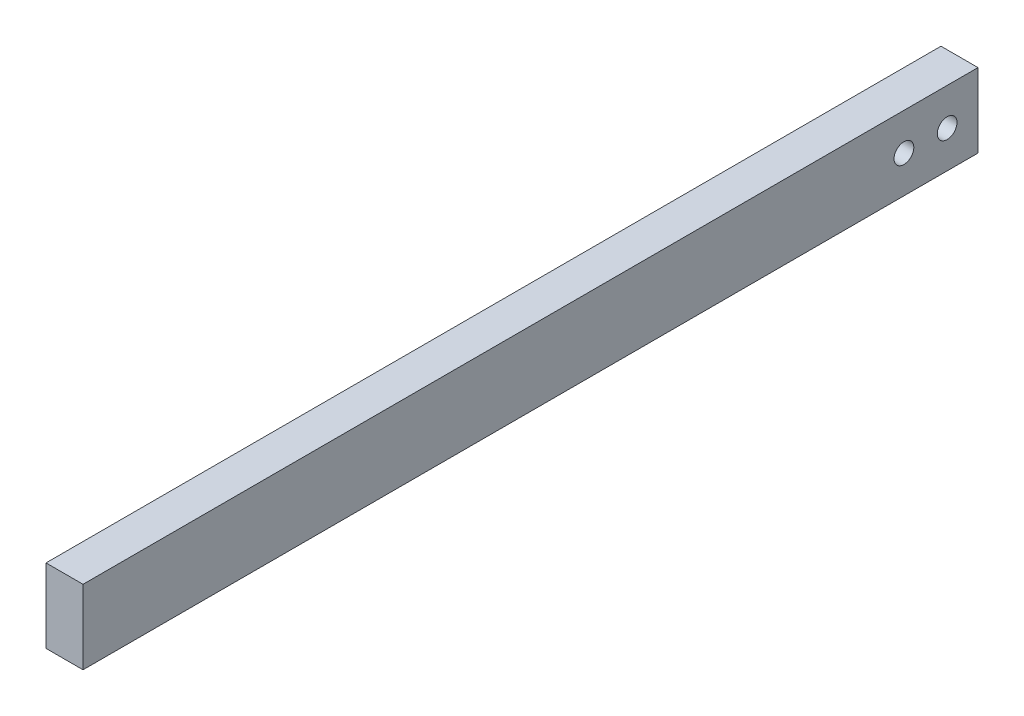
SolidWorks part; units mm, degrees
ref_plane "前视基准面" through (0, 0, 0) normal (0, 0, 1) x (1, 0, 0)
ref_plane "上视基准面" through (0, 0, 0) normal (0, 1, 0) x (1, 0, 0)
ref_plane "右视基准面" through (0, 0, 0) normal (1, 0, 0) x (0, 0, -1)
other "Configuration Table"
sketch "草图1" plane through (0, 0, 0) normal (0, 0, 1) x (1, 0, 0)
  line L1 (-15, -30) -> (15, -30)
  line L2 (-15, -30) -> (-15, 30)
  line L3 (-15, 30) -> (15, 30)
  line L4 (15, -30) -> (15, 30)
  line L5 (0, 30) -> (0, -30) construction
  line L6 (-15, 0) -> (15, 0) construction
  point P0 (0, 0)
  dimension "D1" = 60
  dimension "D2" = 30
extrude "凸台-拉伸1" add sketch "草图1" along normal blind 642
sketch "草图2" plane through (0, 0, 0) normal (0, 0, -1) x (-1, 0, 0)
  line L4 (-15, 30) -> (-15, -30)
  line L5 (-15, -30) -> (15, -30)
  line L6 (15, -30) -> (15, 30)
  line L7 (15, 30) -> (-15, 30)
  line L8 (-15, 30) -> (-15, -30)
  line L9 (-15, -30) -> (15, -30)
  line L10 (15, -30) -> (15, 30)
  line L11 (15, 30) -> (-15, 30)
  dimension "D1" = 0
extrude "凸台-拉伸2" add sketch "草图2" along normal blind 83
sketch "草图3" plane through (-15, 0, 0) normal (-1, 0, 0) x (0, 0, 1)
  line L0 (-83, -30) -> (-83, 30) construction
  line L1 (642, 30) -> (-83, 30) construction
  circle A0 centre (-58, 0) radius 8
  circle A1 centre (-23, 0) radius 8
  dimension "D1" = 16
  dimension "D2" = 16
  dimension "D4" = 35
  dimension "D6" = 30
  dimension "D3" = 25
  dimension "D5" = 30
extrude "切除-拉伸1" cut sketch "草图3" against normal through all
